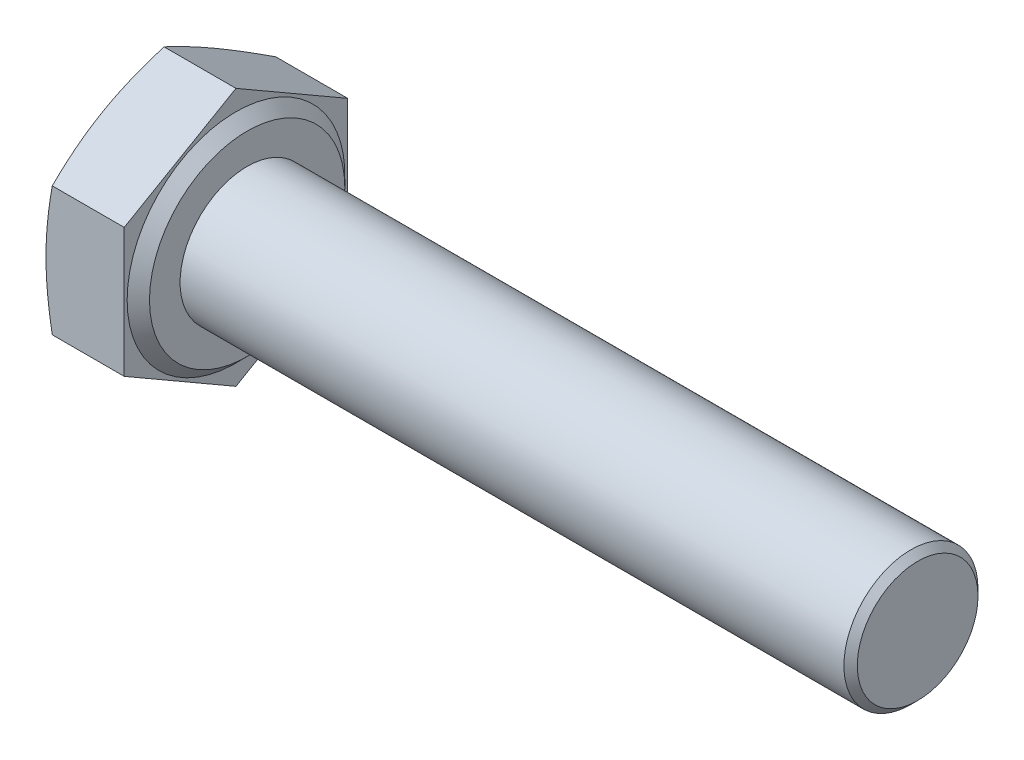
from build123d import *

# Parameters (mm, degrees)
BASEHEAD_DEPTH = 4
SKETCH5_R      = 3
BASEBODY_DEPTH = 30
CHAMFER1_SIZE  = 0.3


with BuildPart() as part:
    # Sketch2 → BaseHead (new body)
    with BuildSketch(Plane(origin=(0, 0, 0), x_dir=(0, 0, -1), z_dir=(1, 0, 0))):
        Polygon((0, -5.773502692), (5, -2.886751346), (5, 2.886751346), (0, 5.773502692), (-5, 2.886751346), (-5, -2.886751346), align=None)
    extrude(amount=BASEHEAD_DEPTH)

    # Sketch3 → BearingFace (revolve, cut)
    with BuildSketch(Plane.XY, mode=Mode.PRIVATE) as bearingface_sk:
        Polygon((4, 5.773502692), (4, 4.37), (3.5, 4.87), (3.5, 5.773502692), align=None)
    revolve(bearingface_sk.sketch.rotate(Axis((-0.957090588, 0, 0), (1, 0, 0)), 90), axis=Axis((-0.957090588, 0, 0), (1, 0, 0)), mode=Mode.SUBTRACT)

    # Sketch4 → HeadChamfer (revolve, cut)
    with BuildSketch(Plane.XY):
        Polygon((0, 5.773502692), (0.281531956, 5.773502692), (0, 5), align=None)
    revolve(axis=Axis((-0.493528746, 0, 0), (1, 0, 0)), mode=Mode.SUBTRACT)

    # Sketch5 → BaseBody (add)
    with BuildSketch(Plane(origin=(4, 0, 0), x_dir=(0, 0, -1), z_dir=(1, 0, 0))):
        Circle(SKETCH5_R)
    extrude(amount=BASEBODY_DEPTH)

    # Chamfer1
    chamfer1_edges = [part.edges().sort_by_distance(p)[0] for p in [
        (34, 0, 3),
    ]]
    chamfer(chamfer1_edges, length=CHAMFER1_SIZE)


solid = part.part
